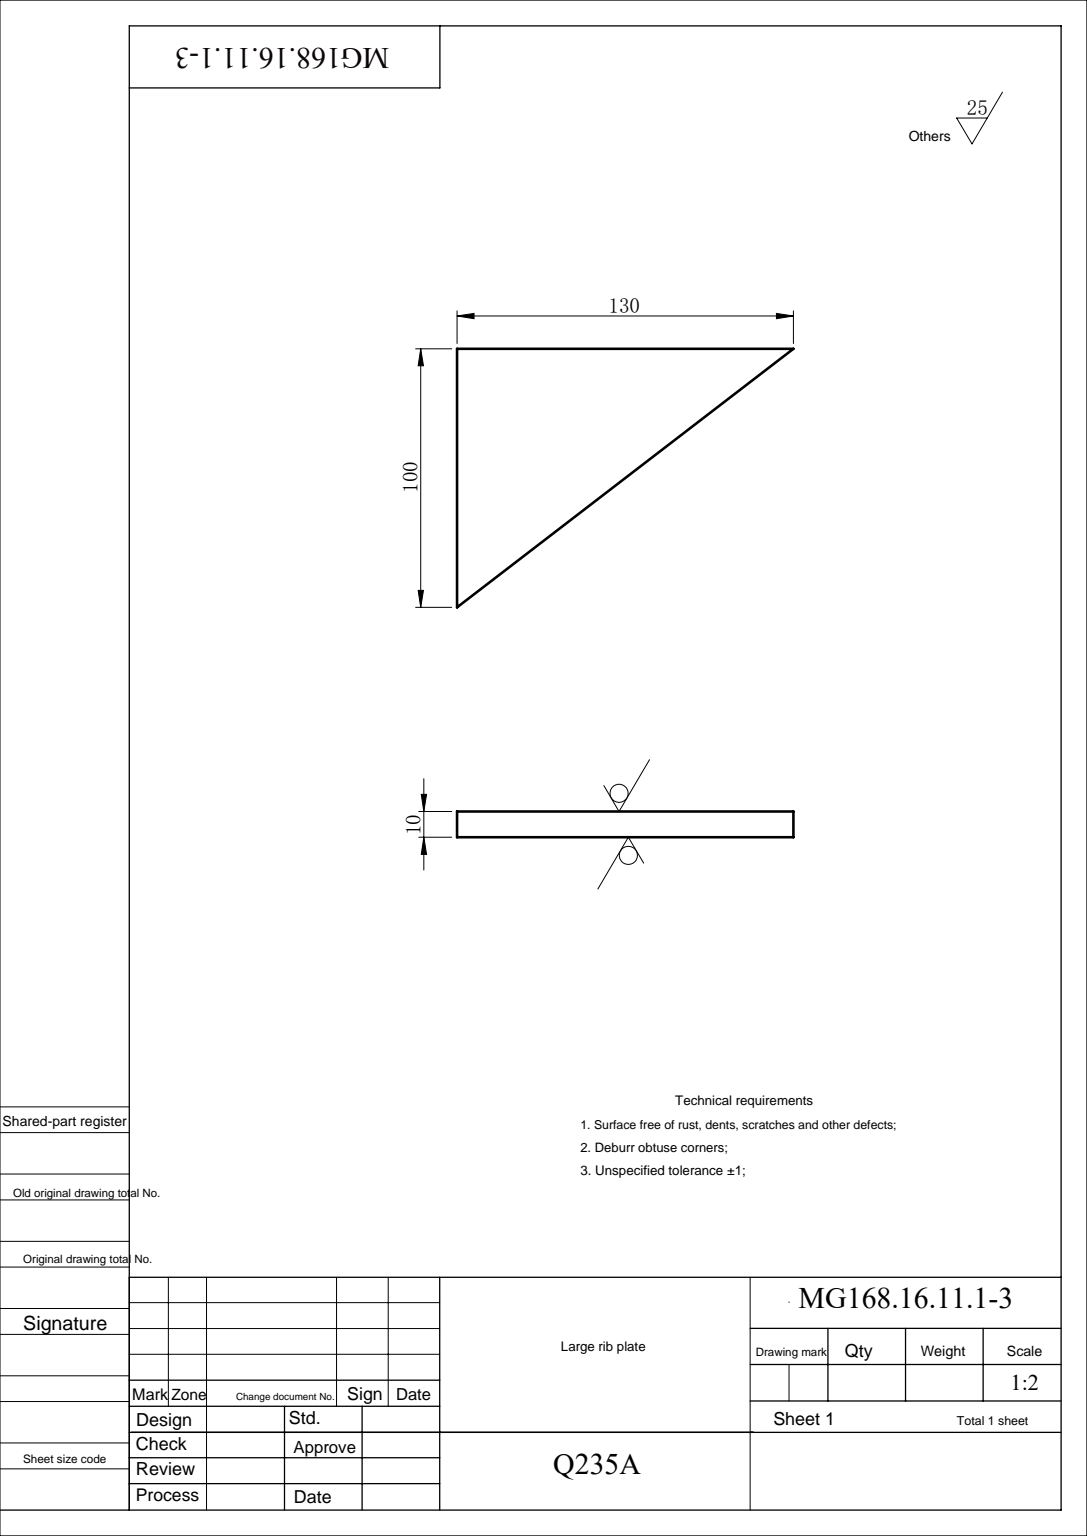
from build123d import *

# Parameters (mm, degrees)
BOSS_EXTRUDE1_DEPTH = 5


with BuildPart() as part:
    # Sketch1 → Boss-Extrude1 (new, symmetric)
    with BuildSketch(Plane(origin=(0, 0, 0), x_dir=(0, 0, -1), z_dir=(1, 0, 0))):
        Polygon((-130, 0), (0, 0), (0, -100), align=None)
    extrude(amount=BOSS_EXTRUDE1_DEPTH, both=True)


solid = part.part
